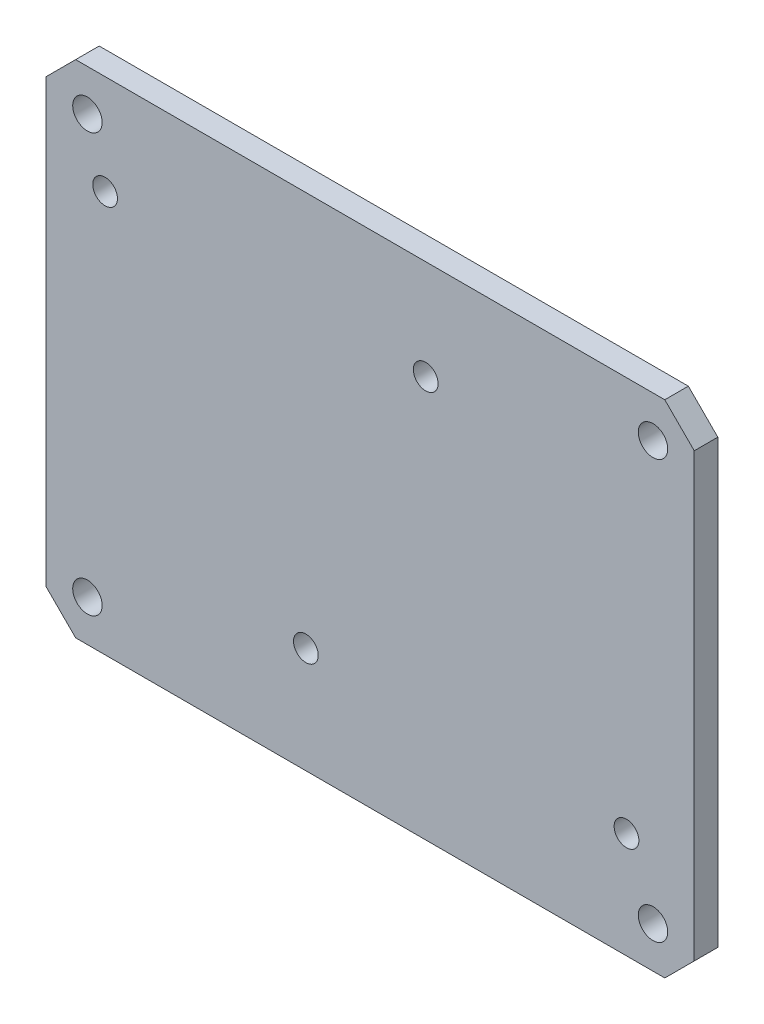
from build123d import *

# Parameters (mm, degrees)
SKETCH_1_W                = 110
SKETCH_1_H                = 85
EXTRUDE_1_DEPTH           = 4
HOLE_WIZARD_M5_1_D        = 4.2
HOLE_WIZARD_M5_1_DEPTH    = 16
HOLE_WIZARD_M5_1_TIP      = 1.2618073
CHAMFER_1_SIZE            = 5
HOLE_WIZARD_5_0_5_1_D     = 5
HOLE_WIZARD_5_0_5_1_DEPTH = 10
HOLE_WIZARD_5_0_5_1_TIP   = 1.443375673


with BuildPart() as part:
    # 草图1 → 凸台-拉伸1 (new body)
    with BuildSketch(Plane.XY):
        with Locations((-21.033643231, -11.115148183)):
            Rectangle(SKETCH_1_W, SKETCH_1_H)
    extrude(amount=EXTRUDE_1_DEPTH)

    # M5 螺纹孔1
    with Locations(Plane.XY.offset(4)):
        with Locations((-66.033643231, 14.494851817), (-31.953643231, -35.615148183), (-11.613643231, 14.494851817), (22.466356769, -35.615148183)):
            Hole(HOLE_WIZARD_M5_1_D / 2, depth=HOLE_WIZARD_M5_1_DEPTH)
            with Locations((0, 0, -(HOLE_WIZARD_M5_1_DEPTH + HOLE_WIZARD_M5_1_TIP / 2))):  # 118° drill point
                Cone(0, HOLE_WIZARD_M5_1_D / 2, HOLE_WIZARD_M5_1_TIP, mode=Mode.SUBTRACT)

    # 倒角1
    chamfer_1_edges = [part.edges().sort_by_distance(p)[0] for p in [
        (-76.033643231, 31.384851817, 2),
        (33.966356769, 31.384851817, 2),
        (33.966356769, -53.615148183, 2),
        (-76.033643231, -53.615148183, 2),
    ]]
    chamfer(chamfer_1_edges, length=CHAMFER_1_SIZE)

    # Ø5.0 (5) 直径孔1
    with Locations(Plane(origin=(0, 0, 0), x_dir=(-1, 0, 0), z_dir=(0, 0, -1))):
        with Locations((69.033643231, 24.384851817), (69.033643231, -46.615148183), (-26.966356769, -46.615148183), (-26.966356769, 24.384851817)):
            Hole(HOLE_WIZARD_5_0_5_1_D / 2, depth=HOLE_WIZARD_5_0_5_1_DEPTH)
            with Locations((0, 0, -(HOLE_WIZARD_5_0_5_1_DEPTH + HOLE_WIZARD_5_0_5_1_TIP / 2))):  # 120° drill point
                Cone(0, HOLE_WIZARD_5_0_5_1_D / 2, HOLE_WIZARD_5_0_5_1_TIP, mode=Mode.SUBTRACT)


solid = part.part
